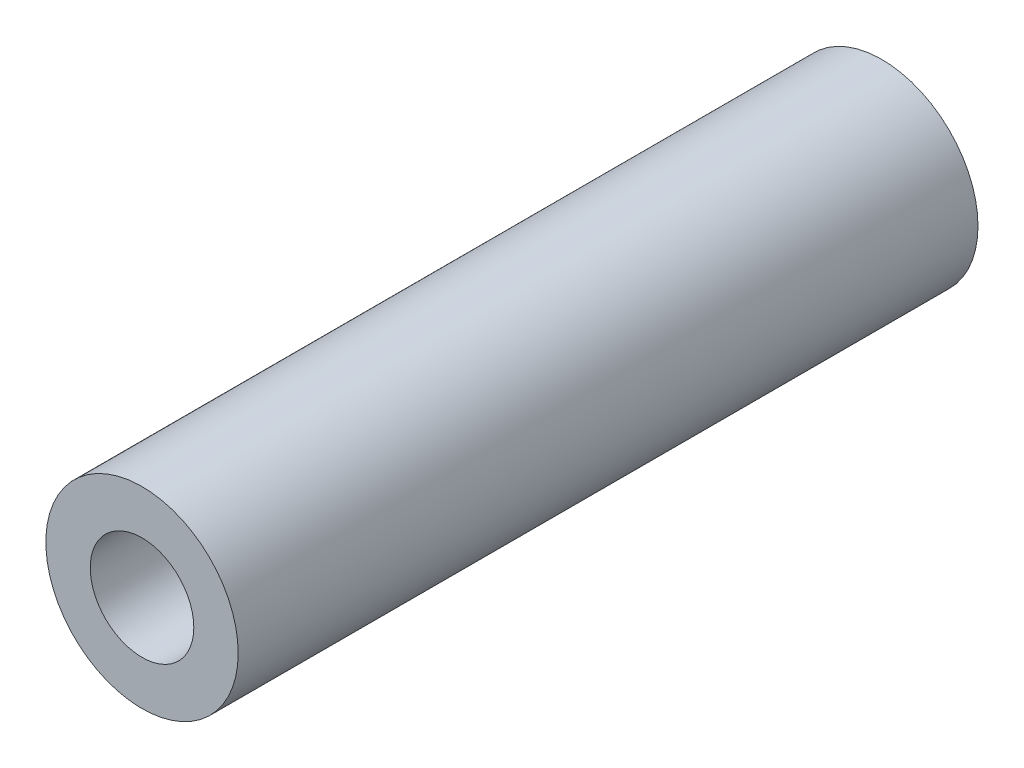
SolidWorks part; units mm, degrees
ref_plane "前视基准面" through (0, 0, 0) normal (0, 0, 1) x (1, 0, 0)
ref_plane "上视基准面" through (0, 0, 0) normal (0, 1, 0) x (1, 0, 0)
ref_plane "右视基准面" through (0, 0, 0) normal (1, 0, 0) x (0, 0, -1)
sketch "草图1" plane through (0, 0, 0) normal (0, 0, 1) x (1, 0, 0)
  circle A0 centre (0, 0) radius 6.5
  circle A1 centre (0, 0) radius 3.5
  dimension "D1" = 7
  dimension "D2" = 13
extrude "凸台-拉伸1" add sketch "草图1" along normal blind 50
